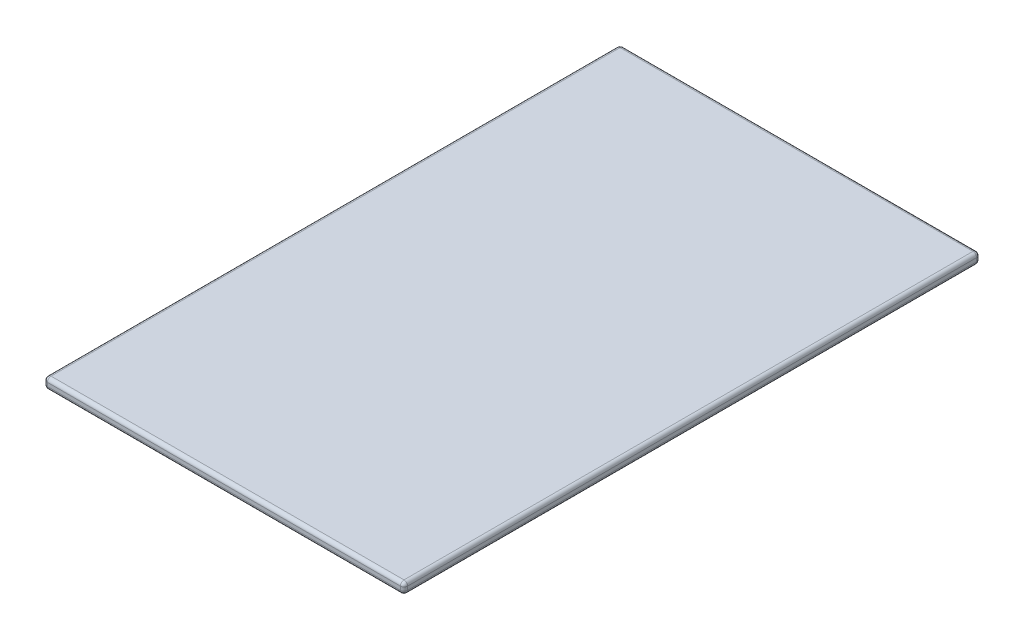
from build123d import *

# Parameters (mm, degrees)
SKETCH1_W           = 1000
SKETCH1_H           = 1600
BOSS_EXTRUDE1_DEPTH = 30
FILLET3_R           = 10


with BuildPart() as part:
    # Sketch1 → Boss-Extrude1 (new body)
    with BuildSketch(Plane(origin=(0, 0, 0), x_dir=(1, 0, 0), z_dir=(0, 1, 0))):
        Rectangle(SKETCH1_W, SKETCH1_H)
    extrude(amount=BOSS_EXTRUDE1_DEPTH)

    # Fillet3
    fillet3_edges = [part.edges().sort_by_distance(p)[0] for p in [
        (-500, 30, 0),
        (0, 30, 800),
        (500, 30, 0),
        (0, 0, 800),
        (-500, 0, 0),
        (0, 0, -800),
        (500, 0, 0),
        (0, 30, -800),
        (500, 15, 800),
        (-500, 15, 800),
        (-500, 15, -800),
        (500, 15, -800),
    ]]
    fillet(fillet3_edges, radius=FILLET3_R)


solid = part.part
